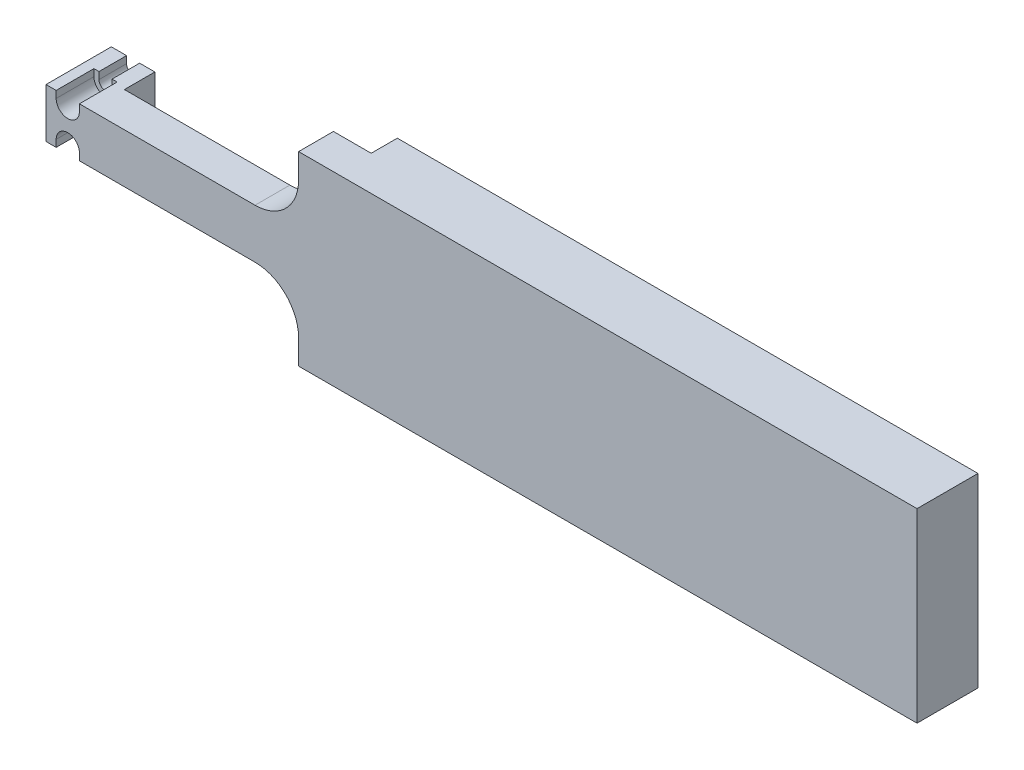
from build123d import *

# Parameters (mm, degrees)
EXTRUDE_1_DEPTH     = 32
SKETCH_2_W          = 87
SKETCH_2_H          = 23.5
CUT_EXTRUDE_1_DEPTH = 22.5
FILLET_1_R          = 15
CUT_EXTRUDE_2_DEPTH = 13
CUT_EXTRUDE_3_REACH = 303.982


with BuildPart() as part:
    # 草图1 → 凸台-拉伸1 (new, symmetric)
    with BuildSketch(Plane(origin=(0, 0, 0), x_dir=(1, 0, 0), z_dir=(0, 1, 0))):
        Polygon((0, 0), (-200, 0), (-200, -9), (-285, -9), (-285, 1.5), (-300, 1.5), (-300, -21), (0, -21), align=None)
    extrude(amount=EXTRUDE_1_DEPTH, both=True)

    # 草图2 → 切除-拉伸1 (cut)
    with BuildSketch(Plane(origin=(0, 0, -1.5), x_dir=(-1, 0, 0), z_dir=(0, 0, -1))):
        with Locations((256.5, -20.25)):
            Rectangle(SKETCH_2_W, SKETCH_2_H)
        with Locations((256.5, 20.25)):
            Rectangle(SKETCH_2_W, SKETCH_2_H)
    extrude(amount=-CUT_EXTRUDE_1_DEPTH, mode=Mode.SUBTRACT)

    # 圆角1
    fillet_1_edges = [part.edges().sort_by_distance(p)[0] for p in [
        (-213, -8.5, 15),
        (-213, 8.5, 15),
    ]]
    fillet(fillet_1_edges, radius=FILLET_1_R)

    # 草图7 → 切除-拉伸2 (cut)
    with BuildSketch(Plane.XY.offset(21)):
        with BuildLine():
            Line((-296.5, 8.5), (-296.5, 6.1))
            ThreePointArc((-296.5, 6.1), (-292.5, 2.1), (-288.5, 6.1))
            Line((-288.5, 6.1), (-288.5, 8.5))
            Line((-288.5, 8.5), (-296.5, 8.5))
        make_face()
    cut_extrude_2 = extrude(amount=-CUT_EXTRUDE_2_DEPTH, mode=Mode.SUBTRACT)

    # 草图8 → 切除-拉伸3 (cut, up to next)
    with BuildSketch(Plane.XY.offset(8), mode=Mode.PRIVATE) as cut_extrude_3_sk1:
        with BuildLine():
            Line((-290.25, 6.1), (-290.25, 8.5))
            Line((-290.25, 8.5), (-294.75, 8.5))
            Line((-294.75, 8.5), (-294.75, 6.1))
            ThreePointArc((-294.75, 6.1), (-292.5, 3.85), (-290.25, 6.1))
        make_face()
    cut_extrude_3_tool1 = extrude(cut_extrude_3_sk1.sketch, amount=-CUT_EXTRUDE_3_REACH, mode=Mode.PRIVATE) & part.part
    cut_extrude_3 = cut_extrude_3_tool1.solids().sort_by_distance((-292.5, 6.386167, 8))[0]
    add(cut_extrude_3, mode=Mode.SUBTRACT)

    # 镜向1: 切除-拉伸2, 切除-拉伸3 across plane
    add(cut_extrude_2.mirror(Plane.ZX), mode=Mode.SUBTRACT)
    add(cut_extrude_3.mirror(Plane.ZX), mode=Mode.SUBTRACT)


solid = part.part
